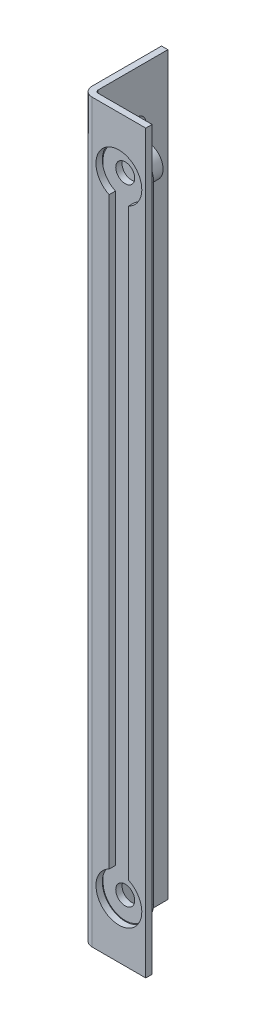
SolidWorks part; units mm, degrees
ref_plane "Front Plane" through (0, 0, 0) normal (0, 0, 1) x (1, 0, 0)
ref_plane "Top Plane" through (0, 0, 0) normal (0, 1, 0) x (1, 0, 0)
ref_plane "Right Plane" through (0, 0, 0) normal (1, 0, 0) x (0, 0, -1)
sketch "Sketch1" plane through (0, 0, 0) normal (0, 1, 0) x (1, 0, 0)
  line L0 (0, 0) -> (-17, 0)
  line L1 (-20, 3) -> (-20, 8.4239)
  line L4 (0, 2) -> (-17, 2)
  line L5 (-18, 3) -> (-18, 8.4239)
  line L9 (0, 2) -> (0, 0)
  line L10 (-19.0962, 11.2912) -> (-13.9038, 18.7088) construction
  line L11 (-17.4577, 10.1443) -> (-12.2654, 17.5619) construction
  line L12 (-11, 21.5761) -> (-11, 37) construction
  line L13 (-13, 21.5761) -> (-13, 37) construction
  line L14 (-20, 8.4239) -> (-20, 25)
  line L15 (-20, 25) -> (-18, 25)
  line L16 (-18, 25) -> (-18, 8.4239)
  arc A2 (-17, 0) -> (-20, 3) centre (-17, 3) cw
  arc A3 (-17, 2) -> (-18, 3) centre (-17, 3) cw
  arc A6 (-13.9038, 18.7088) -> (-13, 21.5761) centre (-18, 21.5761) ccw construction
  arc A7 (-12.2654, 17.5619) -> (-11, 21.5761) centre (-18, 21.5761) ccw construction
  arc A8 (-18, 8.4239) -> (-17.4577, 10.1443) centre (-15, 8.4239) cw construction
  arc A9 (-20, 8.4239) -> (-19.0962, 11.2912) centre (-15, 8.4239) cw construction
  point P14 (-20, 0)
  dimension "D7" = 3
  dimension "D1" = 20
  dimension "D2" = 25
  dimension "D8" = 2
extrude "Boss-Extrude1" add sketch "Sketch1" along normal blind 233
sketch "Sketch2" plane through (-16, 0, 0) normal (1, 0, 0) x (0, 0, -1)
  line L0 (15, 216.35) -> (15, 191.65) construction
  line L1 (18.1, 216.35) -> (18.1, 191.65)
  line L2 (11.9, 216.35) -> (11.9, 191.65)
  line L3 (15, 41.35) -> (15, 16.65) construction
  line L4 (18.1, 41.35) -> (18.1, 16.65)
  line L5 (11.9, 41.35) -> (11.9, 16.65)
  line L8 (25, 233) -> (25, 0) construction
  arc A0 (18.1, 216.35) -> (11.9, 216.35) centre (15, 216.35) ccw
  arc A1 (11.9, 191.65) -> (18.1, 191.65) centre (15, 191.65) ccw
  arc A2 (18.1, 41.35) -> (11.9, 41.35) centre (15, 41.35) ccw
  arc A3 (11.9, 16.65) -> (18.1, 16.65) centre (15, 16.65) ccw
  circle A4 centre (15, 116.1732) radius 3.15
  point P2 (15, 204)
  point P7 (15, 29)
  dimension "D1" = 10
  dimension "D2" = 10
  dimension "D3" = 3.1
  dimension "D4" = 3.1
extrude "Cut-Extrude1" cut sketch "Sketch2" against normal through all
sketch "Sketch3" plane through (0, 0, -2) normal (0, 0, -1) x (-1, 0, 0)
  line L2 (5.4, 208.9462) -> (5.4, 24.0538)
  line L4 (11.6, 208.9462) -> (11.6, 24.0538)
  line L7 (0, 233) -> (0, 0) construction
  arc A0 (11.6, 208.9462) -> (5.4, 208.9462) centre (8.5, 215.5) ccw
  arc A1 (5.4, 24.0538) -> (11.6, 24.0538) centre (8.5, 17.5) ccw
  point P0 (8.5, 116.5)
  dimension "D4" = 14.5
  dimension "D5" = 14.5
  dimension "D1" = 8.5
  dimension "D2" = 3.1
extrude "Cut-Extrude2" cut sketch "Sketch3" against normal through all
sketch "Sketch4" plane through (0, 0, -2) normal (0, 0, -1) x (-1, 0, 0)
  line L0 (0, 233) -> (0, 0) construction
  line L2 (1.5, 215.5) -> (1.5, 17.5)
  line L4 (15.5, 215.5) -> (15.5, 17.5)
  circle A0 centre (8.5, 215.5) radius 3
  circle A1 centre (8.5, 17.5) radius 3
  arc A2 (1.5, 17.5) -> (15.5, 17.5) centre (8.5, 17.5) ccw
  arc A4 (1.5, 215.5) -> (15.5, 215.5) centre (8.5, 215.5) cw
  point P0 (8.5, 107.7004)
  point P11 (0, 116.5)
  dimension "D4" = 6
  dimension "D5" = 6
  dimension "D3" = 0
  dimension "D10" = 7
  dimension "D12" = 7
  dimension "D1" = 14
  dimension "D2" = 8.5
  dimension "D6" = 7
  dimension "D7" = 198
  dimension "D8" = 198
  dimension "D9" = 198
  dimension "D11" = 99
extrude "Boss-Extrude2" add sketch "Sketch4" along normal blind 2
sketch "Sketch5" plane through (0, 0, -4) normal (0, 0, -1) x (-1, 0, 0)
  circle A0 centre (8.5, 215.5) radius 4.9762
extrude "Boss-Extrude3" add sketch "Sketch5" along normal blind 5 separate body
